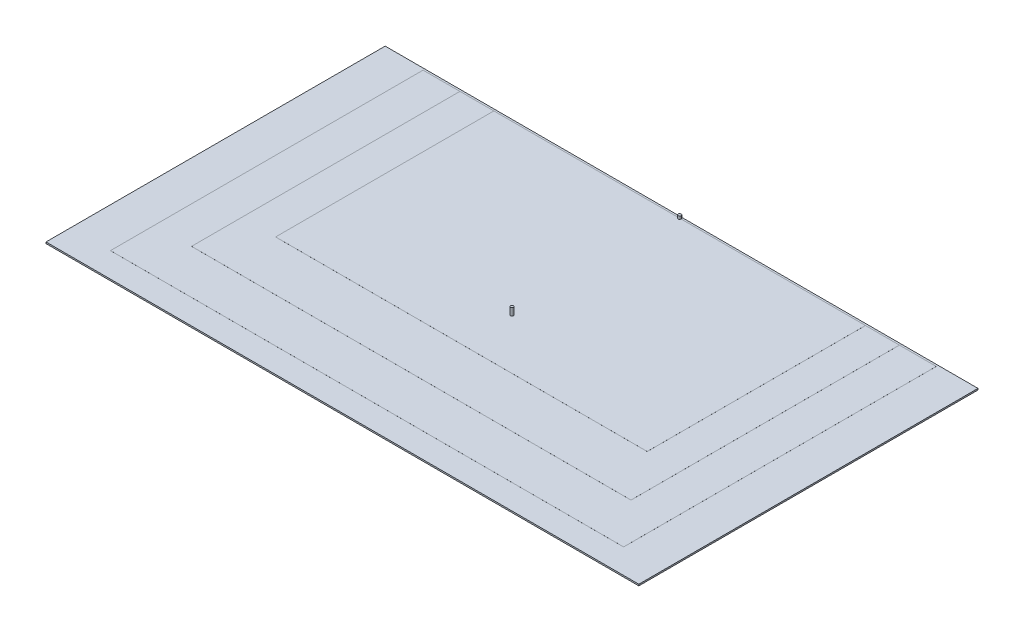
from build123d import *

# Parameters (mm, degrees)
SKETCH_1_W      = 2010
SKETCH_1_H      = 1150
EXTRUDE_1_DEPTH = 2.5
SKETCH_3_W      = 1740
SKETCH_3_H      = 1060
EXTRUDE_5_DEPTH = 0.1
SKETCH_4_W      = 1490
SKETCH_4_H      = 910
EXTRUDE_6_DEPTH = 0.1
SKETCH_5_W      = 1260
SKETCH_5_H      = 740
EXTRUDE_7_DEPTH = 0.1
SKETCH_6_R      = 5
EXTRUDE_8_DEPTH = 25
SKETCH_7_R      = 5
EXTRUDE_9_DEPTH = 10


with BuildPart() as part:
    # 草图1 → 凸台-拉伸1 (new, symmetric)
    with BuildSketch(Plane(origin=(0, 0, 0), x_dir=(1, 0, 0), z_dir=(0, 1, 0))):
        Rectangle(SKETCH_1_W, SKETCH_1_H)
    extrude(amount=EXTRUDE_1_DEPTH, both=True)


with BuildPart() as body_2:
    # 草图3 → 凸台-拉伸5 (new body)
    with BuildSketch(Plane(origin=(0, 2.6, 0), x_dir=(1, 0, 0), z_dir=(0, 1, 0))):
        with Locations((0, 38.5)):
            Rectangle(SKETCH_3_W, SKETCH_3_H)
    extrude(amount=EXTRUDE_5_DEPTH)


with BuildPart() as body_3:
    # 草图4 → 凸台-拉伸6 (new body)
    with BuildSketch(Plane(origin=(0, 2.7, 0), x_dir=(1, 0, 0), z_dir=(0, 1, 0))):
        with Locations((0, 113.5)):
            Rectangle(SKETCH_4_W, SKETCH_4_H)
    extrude(amount=EXTRUDE_6_DEPTH)


with BuildPart() as body_4:
    # 草图5 → 凸台-拉伸7 (new body)
    with BuildSketch(Plane(origin=(0, 2.8, 0), x_dir=(1, 0, 0), z_dir=(0, 1, 0))):
        with Locations((0, 198.5)):
            Rectangle(SKETCH_5_W, SKETCH_5_H)
    extrude(amount=EXTRUDE_7_DEPTH)

    # 草图6 → 凸台-拉伸8 (add, symmetric)
    with BuildSketch(Plane(origin=(0, 2.9, 0), x_dir=(1, 0, 0), z_dir=(0, 1, 0))):
        with Locations(Location((0, 0, 0), (0, 0, 90))):
            Circle(SKETCH_6_R)
    extrude(amount=EXTRUDE_8_DEPTH, both=True)

    # 草图7 → 凸台-拉伸9 (add)
    with BuildSketch(Plane(origin=(0, 2.9, 0), x_dir=(1, 0, 0), z_dir=(0, 1, 0))):
        with Locations(Location((0, 568.5, 0), (0, 0, 180))):
            Circle(SKETCH_7_R)
    extrude(amount=EXTRUDE_9_DEPTH)


solid = Compound([part.part, body_2.part, body_3.part, body_4.part])
